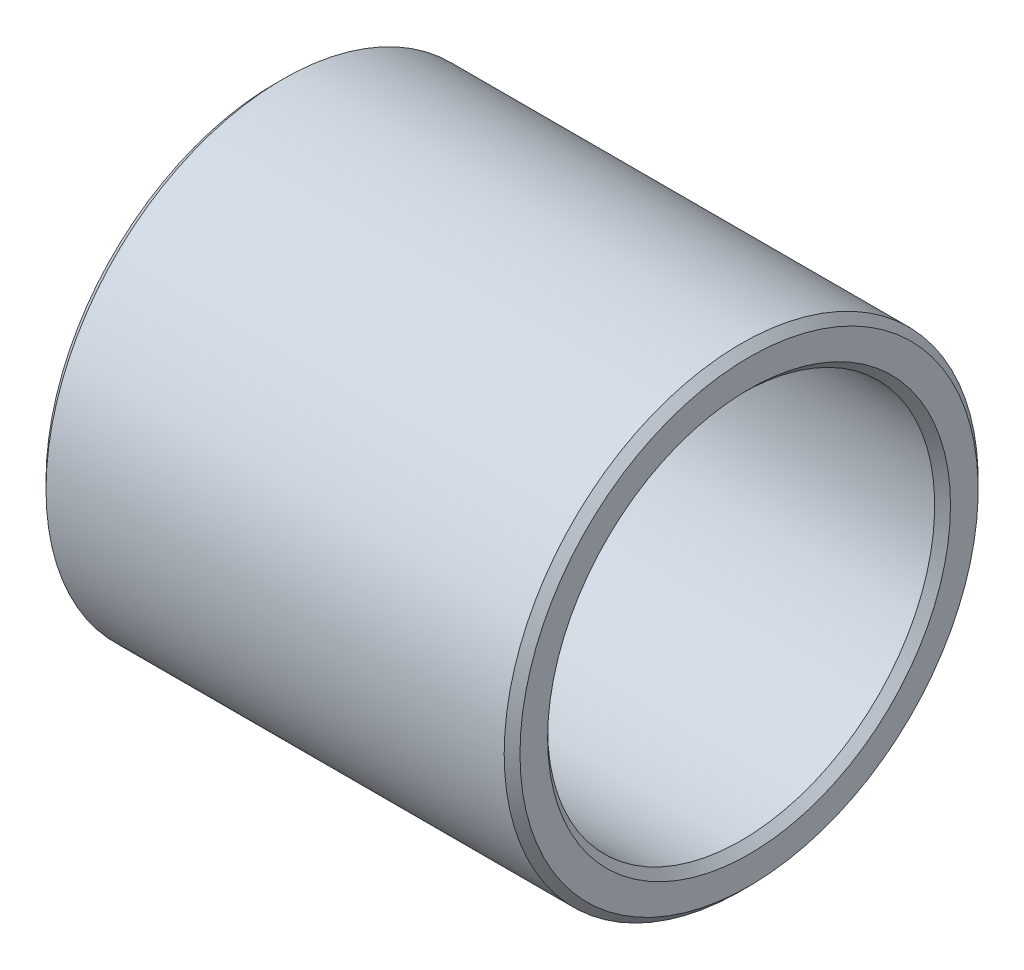
SolidWorks part; units mm, degrees
ref_plane "Front" through (0, 0, 0) normal (0, 0, 1) x (1, 0, 0)
ref_plane "Top" through (0, 0, 0) normal (0, 1, 0) x (1, 0, 0)
ref_plane "Right" through (0, 0, 0) normal (1, 0, 0) x (0, 0, -1)
sketch "草图1" plane through (0, 0, 0) normal (0, 1, 0) x (1, 0, 0)
  line L8 (-15, 14.5) -> (-14.5, 15)
  line L9 (-14.5, 12.25) -> (14.5, 12.25)
  line L10 (-15, 12.75) -> (-15, 14.5)
  line L11 (-14.5, 15) -> (14.5, 15)
  line L12 (15, 12.75) -> (15, 14.5)
  line L13 (-15, 12.25) -> (15, 15) construction
  line L14 (-15, 15) -> (15, 12.25) construction
  line L15 (-15, 12.75) -> (-14.5, 12.25)
  line L16 (14.5, 15) -> (15, 14.5)
  line L17 (14.5, 12.25) -> (15, 12.75)
  line L18 (-1000, 0) -> (49000, 0) construction
  point P0 (0, 13.625)
  dimension "D1" = 12.25
  dimension "D2" = 15
  dimension "D3" = 30
  dimension "D4" = 0
revolve "旋转1" add sketch "草图1" angle 360 about L18
